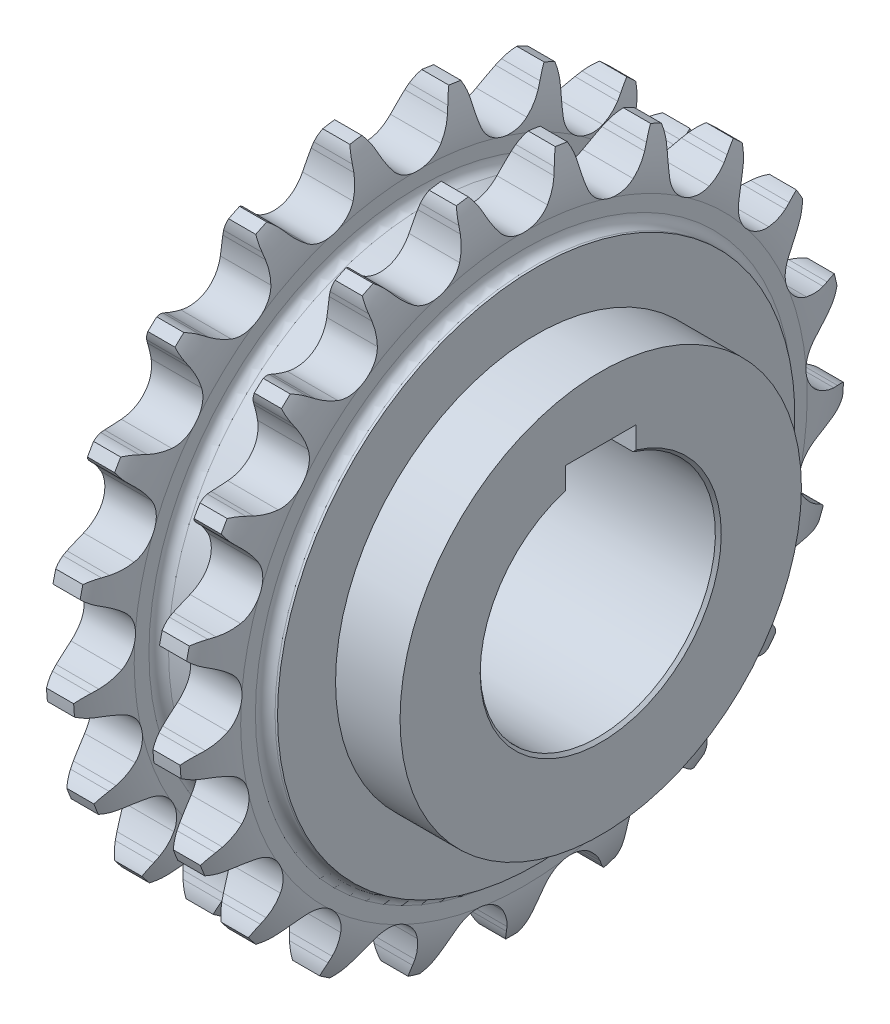
from build123d import *

# Parameters (mm, degrees)
CUT_EXTRUDE_1_DEPTH      = 6.459352492
PATTERN_CIRCULAR_1_COUNT = 21
PATTERN_LINEAR_1_COUNT   = 2
PATTERN_LINEAR_1_PITCH   = 18.11
SKETCH_7_W               = 16.439318006
SKETCH_7_H               = 24
SKETCH_3_W               = 29.081295016
SKETCH_3_H               = 14.131800766
SKETCH_4_W               = 12
SKETCH_4_H               = 4.221215924
CUT_EXTRUDE_2_DEPTH      = 91.212543282
CHAMFER_1_SIZE           = 1
CHAMFER_3_SIZE           = 0.5


with BuildPart() as part:
    # 草图1 → 旋转1 (revolve)
    with BuildSketch(Plane.XY, mode=Mode.PRIVATE) as revolve_1_sk:
        with BuildLine():
            Line((-6.459352492, 20), (-6.459352492, 44))
            Line((-6.459352492, 44), (-6.041681994, 44))
            ThreePointArc((-6.041681994, 44), (-4.860331427, 44.489331427), (-4.371, 45.670681994))
            Line((-4.371, 45.670681994), (-4.371, 48.176704985))
            ThreePointArc((-4.371, 48.176704985), (-3.911774122, 52.480340085), (-2.30725, 56.5))
            Line((-2.30725, 56.5), (2.30725, 56.5))
            ThreePointArc((2.30725, 56.5), (3.911774122, 52.480340085), (4.371, 48.176704985))
            Line((4.371, 48.176704985), (4.371, 45.670681994))
            ThreePointArc((4.371, 45.670681994), (4.860331427, 44.489331427), (6.041681994, 44))
            Line((6.041681994, 44), (6.459352492, 44))
            Line((6.459352492, 44), (6.459352492, 20))
            Line((6.459352492, 20), (-6.459352492, 20))
        make_face()
    revolve(revolve_1_sk.sketch.rotate(Axis((-7.9375, 0, 0), (1, 0, 0)), 90), axis=Axis((-7.9375, 0, 0), (1, 0, 0)))

    # 草图2 → 切除-拉伸1 (cut, symmetric)
    with BuildSketch(Plane(origin=(0, 0, 0), x_dir=(0, 0, -1), z_dir=(1, 0, 0))):
        with BuildLine():
            Line((5.852739584, 53.156379816), (6.249341137, 54.112736402))
            ThreePointArc((6.249341137, 54.112736402), (6.752605781, 55.10660921), (7.399855354, 56.013321101))
            ThreePointArc((7.399855354, 56.013321101), (0, 56.5), (-7.399855354, 56.013321101))
            ThreePointArc((-7.399855354, 56.013321101), (-6.752605781, 55.10660921), (-6.249341137, 54.112736402))
            Line((-6.249341137, 54.112736402), (-5.852739584, 53.156379816))
            ThreePointArc((-5.852739584, 53.156379816), (-5.064210074, 51.564909521), (-4.070411778, 50.09286284))
            ThreePointArc((-4.070411778, 50.09286284), (0, 48.101304985), (4.070411778, 50.09286284))
            ThreePointArc((4.070411778, 50.09286284), (5.064210074, 51.564909521), (5.852739584, 53.156379816))
        make_face()
    cut_extrude_1 = extrude(amount=CUT_EXTRUDE_1_DEPTH, both=True, mode=Mode.SUBTRACT)

    # 阵列(圆周)1: 切除-拉伸1 ×21 about axis
    pattern_circular_1_axis = Axis((0, 0, 0), (1, 0, 0))
    for i in range(1, PATTERN_CIRCULAR_1_COUNT):
        add(cut_extrude_1.rotate(pattern_circular_1_axis, i * 360 / PATTERN_CIRCULAR_1_COUNT), mode=Mode.SUBTRACT)


with BuildPart() as pattern_linear_1_1:
    # 阵列(线性)1: pattern copy
    add(part.part.moved(Location(Vector(1, 0, 0) * (1 * PATTERN_LINEAR_1_PITCH))))


with BuildPart() as part_1:
    add(part.part)

    add(pattern_linear_1_1.part)  # 旋转4 merges 阵列(线性)1_1
    # 草图7 → 旋转4 (revolve)
    with BuildSketch(Plane.XY, mode=Mode.PRIVATE) as revolve_4_sk:
        with Locations((14.679011495, 32)):
            Rectangle(SKETCH_7_W, SKETCH_7_H)
    revolve(revolve_4_sk.sketch.rotate(Axis((0, 0, 0), (1, 0, 0)), 90), axis=Axis((0, 0, 0), (1, 0, 0)))

    # 草图3 → 旋转2 (revolve)
    with BuildSketch(Plane.XY, mode=Mode.PRIVATE) as revolve_2_sk:
        with Locations((21, 27.065900383)):
            Rectangle(SKETCH_3_W, SKETCH_3_H)
    revolve(revolve_2_sk.sketch.rotate(Axis((0, 0, 0), (1, 0, 0)), 90), axis=Axis((0, 0, 0), (1, 0, 0)))

    # 草图4 → 切除-拉伸2 (cut, through all)
    with BuildSketch(Plane.ZY.offset(6.459352492)):
        with Locations((0, 21.18939199)):
            Rectangle(SKETCH_4_W, SKETCH_4_H)
    extrude(amount=-CUT_EXTRUDE_2_DEPTH, mode=Mode.SUBTRACT)

    # 倒角1
    chamfer_1_edges = [part_1.edges().sort_by_distance(p)[0] for p in [
        (-6.459352492, -20, 0),
    ]]
    chamfer(chamfer_1_edges, length=CHAMFER_1_SIZE)

    # 倒角3
    chamfer_3_edges = [part_1.edges().sort_by_distance(p)[0] for p in [
        (35.540647508, -20, 0),
    ]]
    chamfer(chamfer_3_edges, length=CHAMFER_3_SIZE)


solid = part_1.part
